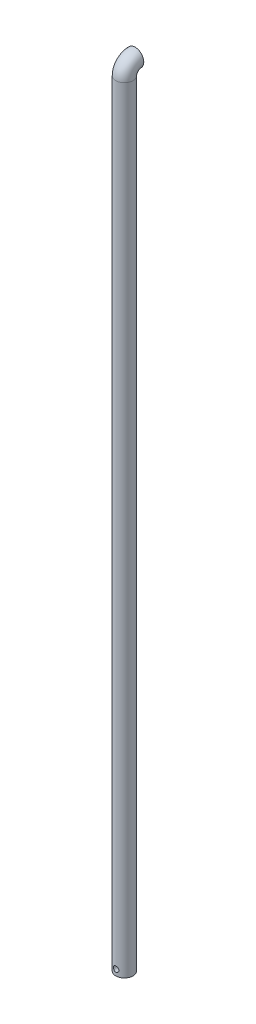
SolidWorks part; units mm, degrees
material "Q235B"
ref_plane "Front Plane" through (0, 0, 0) normal (0, 0, 1) x (1, 0, 0)
ref_plane "Top Plane" through (0, 0, 0) normal (0, 1, 0) x (1, 0, 0)
ref_plane "Right Plane" through (0, 0, 0) normal (1, 0, 0) x (0, 0, -1)
sketch "Sketch1" plane through (0, 0, 0) normal (0, 0, 1) x (1, 0, 0)
  circle A0 centre (0, 0) radius 8
  circle A1 centre (0, 0) radius 3
  dimension "D1" = 16
  dimension "D2" = 6
sketch "Sketch2" plane through (0, 0, 0) normal (1, 0, 0) x (0, 0, -1)
  line L0 (0, 0) -> (-0.05, 0)
  line L1 (-10, -9.95) -> (-10, -730)
  arc A0 (-0.05, 0) -> (-10, -9.95) centre (-0.05, -9.95) ccw
  point P6 (-10, 0)
  dimension "D3" = 9.95
  dimension "D1" = 10
  dimension "D2" = 730
sweep "Sweep1" add profiles "Sketch1" path "Sketch2"
sketch "Sketch3" plane through (0, -730, 0) normal (0, -1, 0) x (1, 0, 0)
  circle A0 centre (0, 10) radius 3
  dimension "D1" = 6
extrude "Boss-Extrude1" add sketch "Sketch3" against normal blind 3
sketch "Sketch4" plane through (0, 0, 0) normal (0, 0, 1) x (1, 0, 0)
  line L0 (-8, -730) -> (8, -730) construction
  line L1 (8, -730) -> (8, -9.95) construction
  circle A0 centre (0, -724.5) radius 2.5
  dimension "D1" = 5
  dimension "D3" = 8
  dimension "D2" = 5.5
extrude "Cut-Extrude2" cut sketch "Sketch4" against normal through all and the other way through all
